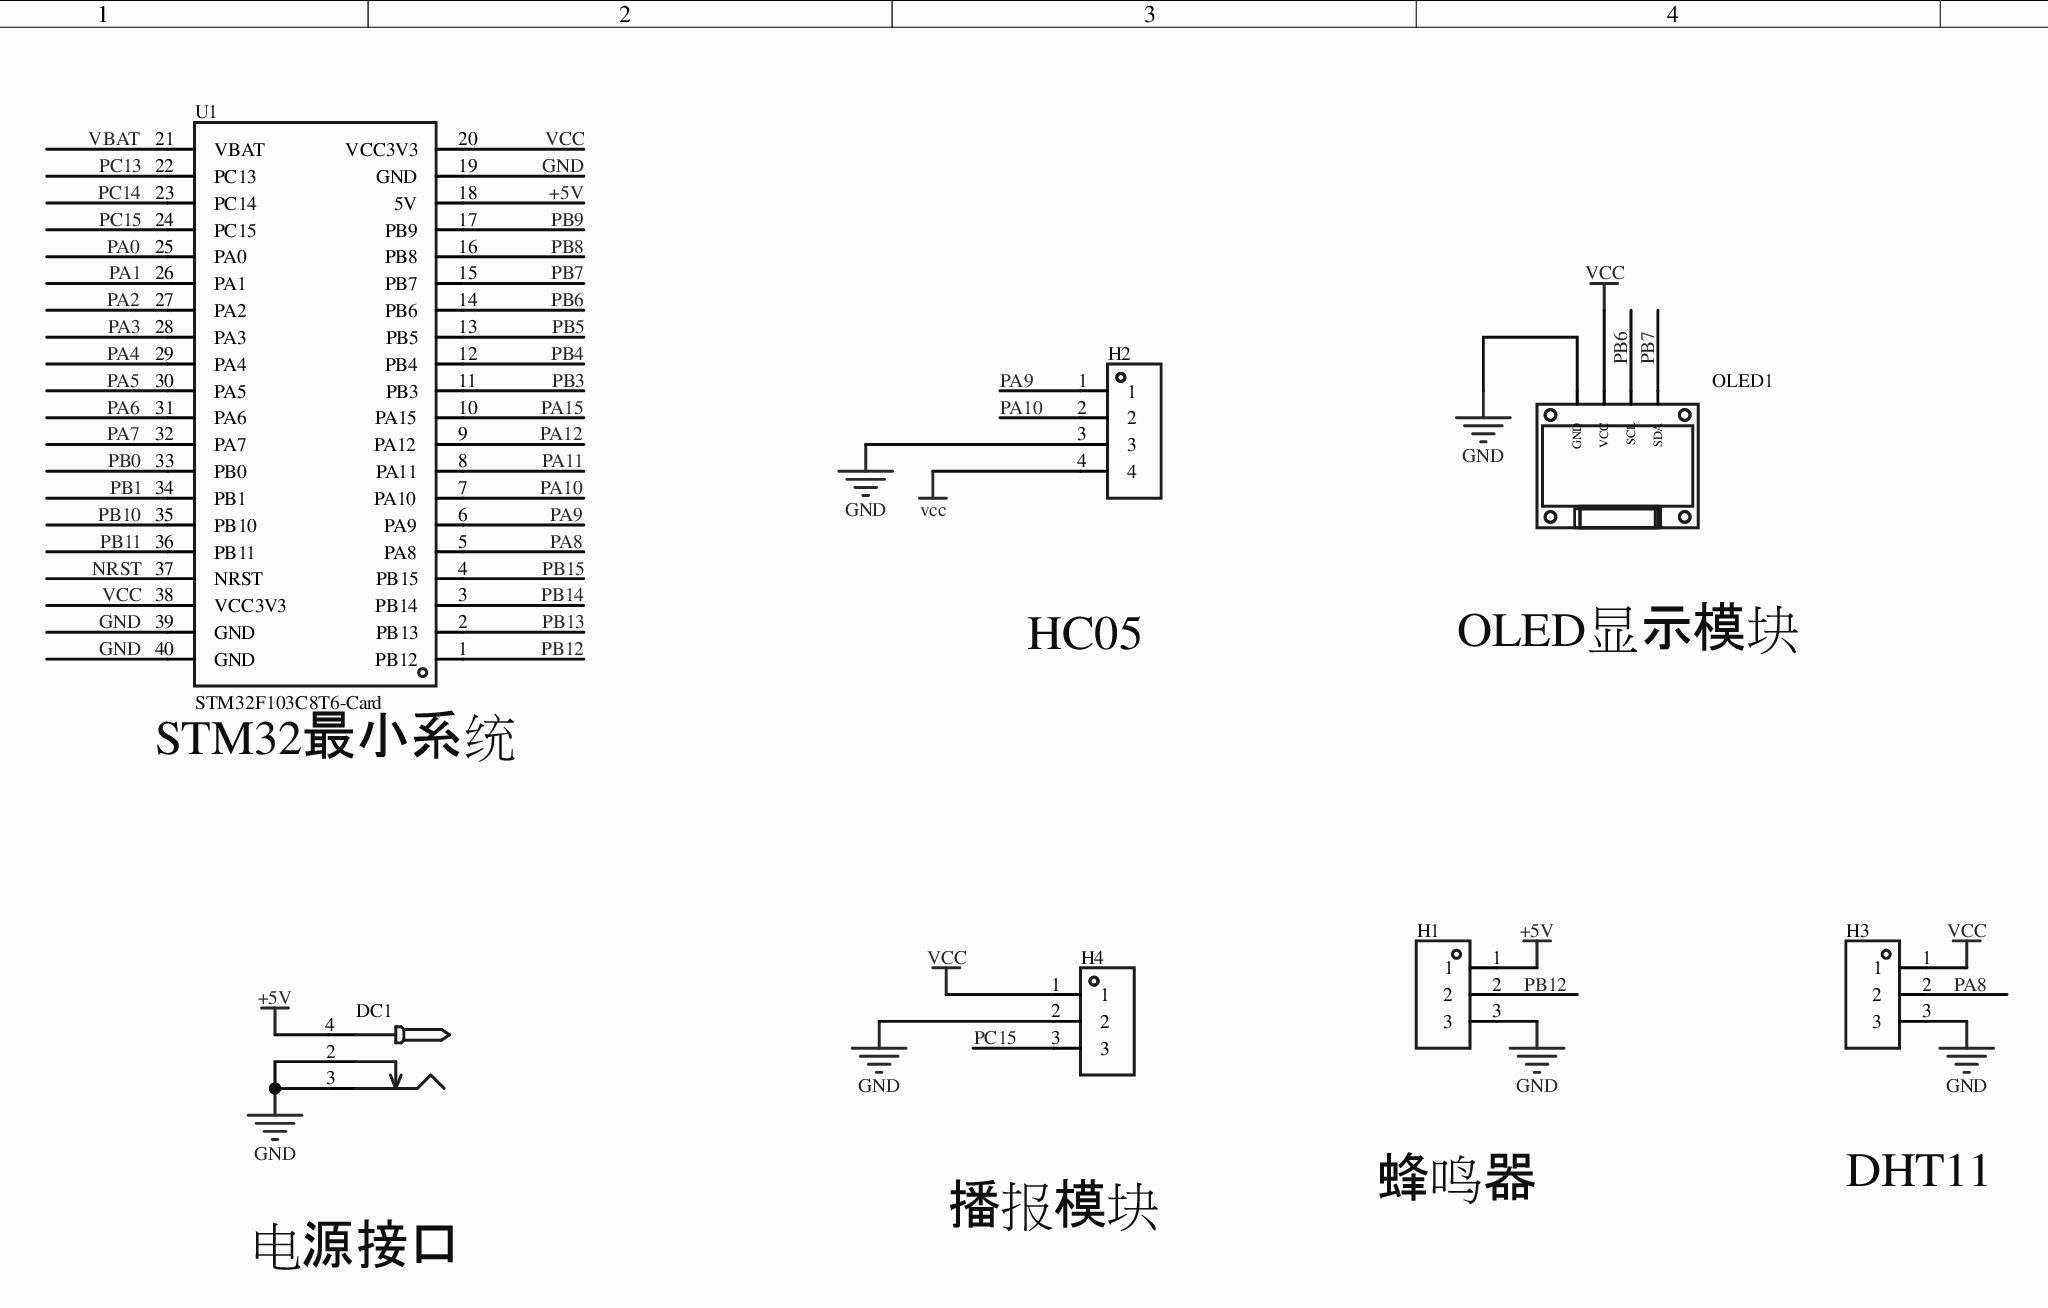
[diagram p0: MISC51802-3.schdoc]
# Altium project MISC51802-2.PrjPcb
1 sheet, 7 parts. Net scope: global (net labels, ports and power ports of the same name join across sheets).
Board file: MISC51802.pcbdoc

## Sheet MISC51802-3.schdoc
size 297 x 209 mm; Version: V1.0; @Project Name: MISC51802; @Page Count: 1; @Update Date: 2026-04-27; @Create Date: 2026-04-27; @Schematic Name: MISC51802; @Page No: 1; @Create Time: 23:22:16; @Update Time: 17:32:40; @Board Name: MISC51802

### Parts
DC1  (no value)  [DC-2.0]
H1  (no value)  [HDR-TH_3P-P2.54-V-F]
H2  (no value)  [HDR-TH_4P-P2.54-V-F]
H3  (no value)  [HDR-TH_3P-P2.54-V-F]
H4  (no value)  [HDR-TH_3P-P2.54-V-M]
OLED1  (no value)  [0.96OLED_4P]
U1  STM32F103C8T6-Card  [CONN-TH_L53.3-W22.9_STM32F103C8T6-CARD]

### Nets
+5V: DC1.4 H1.1 U1.18(5V)
GND: DC1.2 DC1.3 H1.3 H2.3 H3.3 H4.2 OLED1.1(GND) U1.19(GND) U1.39(GND) U1.40(GND)
VCC: H2.4 H3.1 H4.1 OLED1.2(VCC) U1.20(VCC3V3) U1.38(VCC3V3)
NRST: U1.37(NRST)
PA0: U1.25(PA0)
PA1: U1.26(PA1)
PA2: U1.27(PA2)
PA3: U1.28(PA3)
PA4: U1.29(PA4)
PA5: U1.30(PA5)
PA6: U1.31(PA6)
PA7: U1.32(PA7)
PA8: H3.2 U1.5(PA8)
PA9: H2.1 U1.6(PA9)
PA10: H2.2 U1.7(PA10)
PA11: U1.8(PA11)
PA12: U1.9(PA12)
PA15: U1.10(PA15)
PB0: U1.33(PB0)
PB1: U1.34(PB1)
PB3: U1.11(PB3)
PB4: U1.12(PB4)
PB5: U1.13(PB5)
PB6: OLED1.3(SCL) U1.14(PB6)
PB7: OLED1.4(SDA) U1.15(PB7)
PB8: U1.16(PB8)
PB9: U1.17(PB9)
PB10: U1.35(PB10)
PB11: U1.36(PB11)
PB12: H1.2 U1.1(PB12)
PB13: U1.2(PB13)
PB14: U1.3(PB14)
PB15: U1.4(PB15)
PC13: U1.22(PC13)
PC14: U1.23(PC14)
PC15: H4.3 U1.24(PC15)
VBAT: U1.21(VBAT)

### Notes on the sheet
- HC05
- OLED显示模块
- (near U1) STM32最小系统
- 蜂鸣器
- DHT11
- 电源接口
- 播报模块

### Library data of the parts
DC1 = DC-005_2.0: Symbol: DC电源接口; ConvertToPcb: yes; ModelId: f5f20b8a2308479b936ba3c2698865bb0819f05c4eef4c71ace90d822a990e87; ModelName: DC-IN-TH_DC-5520-1; ModelTransform: 372.05,551.18,582.68,90,0,0,137.8,0,-149.61; Device: DC-005_2.0; AddInBom: yes; Supplier Footprint: 插件; FootprintName: DC-2.0
H1 H3 = HDR-F_2.54_1x3P: Symbol: PM254V-11-03-H85; 3D Model: f3b3cc5aae9641bf9e56fc160cef875b; 3D Model Transform: 299.9994,100,0,0,0,0,0,0,-118.11; ConvertToPcb: yes; ModelName: HDR2.54-F-LI-1X3P; Device: HDR-F_2.54_1x3P; Supplier Part: C541850; Supplier Footprint: 插件; FootprintName: HDR-TH_3P-P2.54-V-F; AddInBom: yes
H2 = HDR-F_2.54_1x4P: Symbol: 2.54-1*4P母; ConvertToPcb: yes; ModelId: d187812051054f85879fcaa51a310d8e0819f05c4eef4c71ace90d822a990e87; ModelTransform: 419.6842,98.464,0,0,0,0,0,0,-118.11; Device: HDR-F_2.54_1x4P; FootprintName: HDR-TH_4P-P2.54-V-F; AddInBom: yes; SupplierPart: C2718488; Supplier Footprint: 插件; ModelName: HDR-TH_4P-P2.54-V-F
H4 = HDR-M_2.54_1x3P: AddInBom: yes; ModelId: bb473b6d38ff42a99216a4fcdbdcc4cb0819f05c4eef4c71ace90d822a990e87; ModelName: HDR-TH_3P-P2.54-M-LI-1X3P; ModelTransform: 300.03877,100,0,0,0,0,0,0,-118.11; Symbol: HDR-M_2.54_1x3P; Device: HDR-M_2.54_1x3P; ConvertToPcb: yes; FootprintName: HDR-TH_3P-P2.54-V-M; SupplierPart: C2937625; Supplier Footprint: 插件
OLED1 = 0.96OLED模块_4P: ConvertToPcb: yes; ModelId: 79c000fdb68d45a296c2e9bedf4f9055; ModelTransform: 1393.69792,1318.895,0,0,0,0,0,-560.079,-137.795; Device: 0.96OLED模块_4P; Symbol: 0.96OLED模块_4P; FootprintName: 0.96OLED_4P; AddInBom: yes; Supplier Footprint: 插件; ModelName: 0.96OLED_4P
U1 = STM32F103C8T6-Card: AddInBom: yes; Device: STM32F103C8T6-Card; Symbol: STM32F103C8T6-CARD; FootprintName: CONN-TH_L53.3-W22.9_STM32F103C8T6-CARD; LCSC Part Name: STM32F103C8T6-Card; SupplierPart: C9900077949; ManufacturerPart: STM32F103C8T6-Card; Supplier Footprint: 插件; Supplier: LCSC; ConvertToPcb: yes